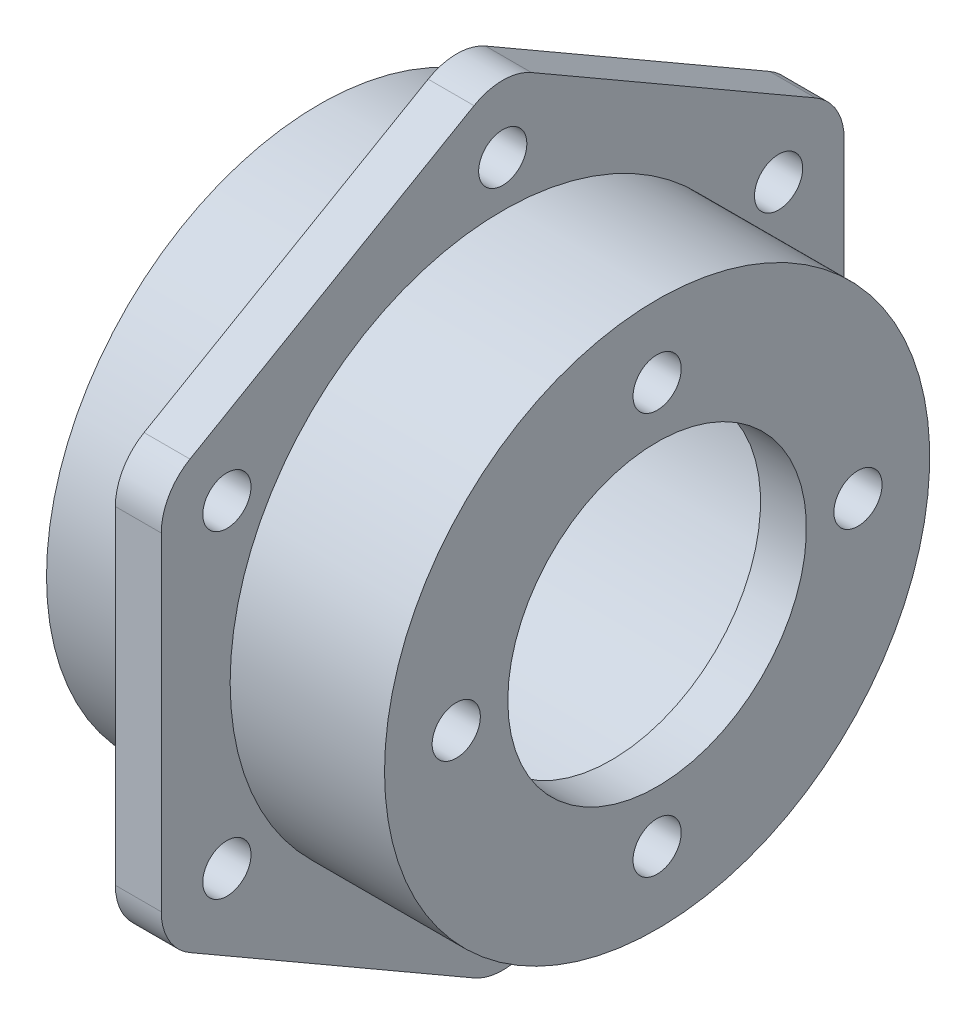
from build123d import *

# Parameters (mm, degrees)
SKETCH_2_R          = 2.1
CUT_EXTRUDE_1_DEPTH = 48.333920184
SKETCH_3_R          = 2.1
CUT_EXTRUDE_2_DEPTH = 53.389073288
EXTRUDE_1_DEPTH     = 4
FILLET_1_R          = 5


with BuildPart() as part:
    # 草图1 → 旋转1 (revolve)
    with BuildSketch(Plane(origin=(0, 0, 0), x_dir=(1, 0, 0), z_dir=(0, 1, 0)), mode=Mode.PRIVATE) as revolve_1_sk:
        Polygon((0, 21.25), (0, 23.75), (12, 23.75), (12, 31.5), (16, 31.5), (16, 23.75), (29.45, 23.75), (29.45, 13.01), (25.45, 13.01), (25.45, 21.25), align=None)
    revolve(revolve_1_sk.sketch.rotate(Axis((-873.269597079, 0, 0), (1, 0, 0)), 180), axis=Axis((-873.269597079, 0, 0), (1, 0, 0)))

    # 草图2 → 切除-拉伸1 (cut, through all)
    with BuildSketch(Plane(origin=(16, 0, 0), x_dir=(0, 0, -1), z_dir=(1, 0, 0))):
        with Locations((0, 27.75)):
            Circle(SKETCH_2_R)
        with Locations((-24.032204955, 13.875)):
            Circle(SKETCH_2_R)
        with Locations((-24.032204955, -13.875)):
            Circle(SKETCH_2_R)
        with Locations((0, -27.75)):
            Circle(SKETCH_2_R)
        with Locations((24.032204955, -13.875)):
            Circle(SKETCH_2_R)
        with Locations((24.032204955, 13.875)):
            Circle(SKETCH_2_R)
        with BuildLine():
            ThreePointArc((31.5, 0), (31.059418861, 5.25), (29.75, 10.35313962))
            Line((29.75, 10.35313962), (29.75, -10.35313962))
            ThreePointArc((29.75, -10.35313962), (31.059418861, -5.25), (31.5, 0))
        make_face()
        with BuildLine():
            ThreePointArc((23.84108192, 20.587685952), (15.75, 27.279800219), (5.90891808, 30.940825573))
            Line((5.90891808, 30.940825573), (23.84108192, 20.587685952))
        make_face()
        with BuildLine():
            Line((-23.84108192, 20.587685952), (-5.90891808, 30.940825573))
            ThreePointArc((-5.90891808, 30.940825573), (-15.75, 27.279800219), (-23.84108192, 20.587685952))
        make_face()
        with BuildLine():
            Line((-29.75, -10.35313962), (-29.75, 10.35313962))
            ThreePointArc((-29.75, 10.35313962), (-31.5, 0), (-29.75, -10.35313962))
        make_face()
        with BuildLine():
            Line((-5.90891808, -30.940825573), (-23.84108192, -20.587685952))
            ThreePointArc((-23.84108192, -20.587685952), (-15.75, -27.279800219), (-5.90891808, -30.940825573))
        make_face()
        with BuildLine():
            ThreePointArc((5.90891808, -30.940825573), (15.75, -27.279800219), (23.84108192, -20.587685952))
            Line((23.84108192, -20.587685952), (5.90891808, -30.940825573))
        make_face()
    extrude(amount=-CUT_EXTRUDE_1_DEPTH, mode=Mode.SUBTRACT)

    # 草图3 → 切除-拉伸2 (cut, through all)
    with BuildSketch(Plane(origin=(29.45, 0, 0), x_dir=(0, 0, -1), z_dir=(1, 0, 0))):
        with Locations((0, 17.5)):
            Circle(SKETCH_3_R)
        with Locations((17.5, 0)):
            Circle(SKETCH_3_R)
        with Locations((0, -17.5)):
            Circle(SKETCH_3_R)
        with Locations((-17.5, 0)):
            Circle(SKETCH_3_R)
    extrude(amount=-CUT_EXTRUDE_2_DEPTH, mode=Mode.SUBTRACT)

    # 草图2<3> → 凸台-拉伸1 (add)
    with BuildSketch(Plane(origin=(16, 0, 0), x_dir=(0, 0, -1), z_dir=(1, 0, 0))):
        with BuildLine():
            ThreePointArc((-29.75, 10.35313962), (-27.279800219, 15.75), (-23.84108192, 20.587685952))
            Line((-23.84108192, 20.587685952), (-29.75, 17.176170508))
            Line((-29.75, 17.176170508), (-29.75, 10.35313962))
        make_face()
        with BuildLine():
            Line((5.90891808, 30.940825573), (0, 34.352341017))
            Line((0, 34.352341017), (-5.90891808, 30.940825573))
            ThreePointArc((-5.90891808, 30.940825573), (0, 31.5), (5.90891808, 30.940825573))
        make_face()
        with BuildLine():
            Line((29.75, 17.176170508), (23.84108192, 20.587685952))
            ThreePointArc((23.84108192, 20.587685952), (27.279800219, 15.75), (29.75, 10.35313962))
            Line((29.75, 10.35313962), (29.75, 17.176170508))
        make_face()
        with BuildLine():
            Line((29.75, -17.176170508), (29.75, -10.35313962))
            ThreePointArc((29.75, -10.35313962), (27.279800219, -15.75), (23.84108192, -20.587685952))
            Line((23.84108192, -20.587685952), (29.75, -17.176170508))
        make_face()
        with BuildLine():
            ThreePointArc((5.90891808, -30.940825573), (0, -31.5), (-5.90891808, -30.940825573))
            Line((-5.90891808, -30.940825573), (0, -34.352341017))
            Line((0, -34.352341017), (5.90891808, -30.940825573))
        make_face()
        with BuildLine():
            ThreePointArc((-23.84108192, -20.587685952), (-27.279800219, -15.75), (-29.75, -10.35313962))
            Line((-29.75, -10.35313962), (-29.75, -17.176170508))
            Line((-29.75, -17.176170508), (-23.84108192, -20.587685952))
        make_face()
    extrude(amount=-EXTRUDE_1_DEPTH)

    # 圆角1
    fillet_1_edges = [part.edges().sort_by_distance(p)[0] for p in [
        (14, -17.176170508, 29.75),
        (14, -34.352341017, 0),
        (14, -17.176170508, -29.75),
        (14, 17.176170508, -29.75),
        (14, 34.352341017, 0),
        (14, 17.176170508, 29.75),
    ]]
    fillet(fillet_1_edges, radius=FILLET_1_R)


solid = part.part
